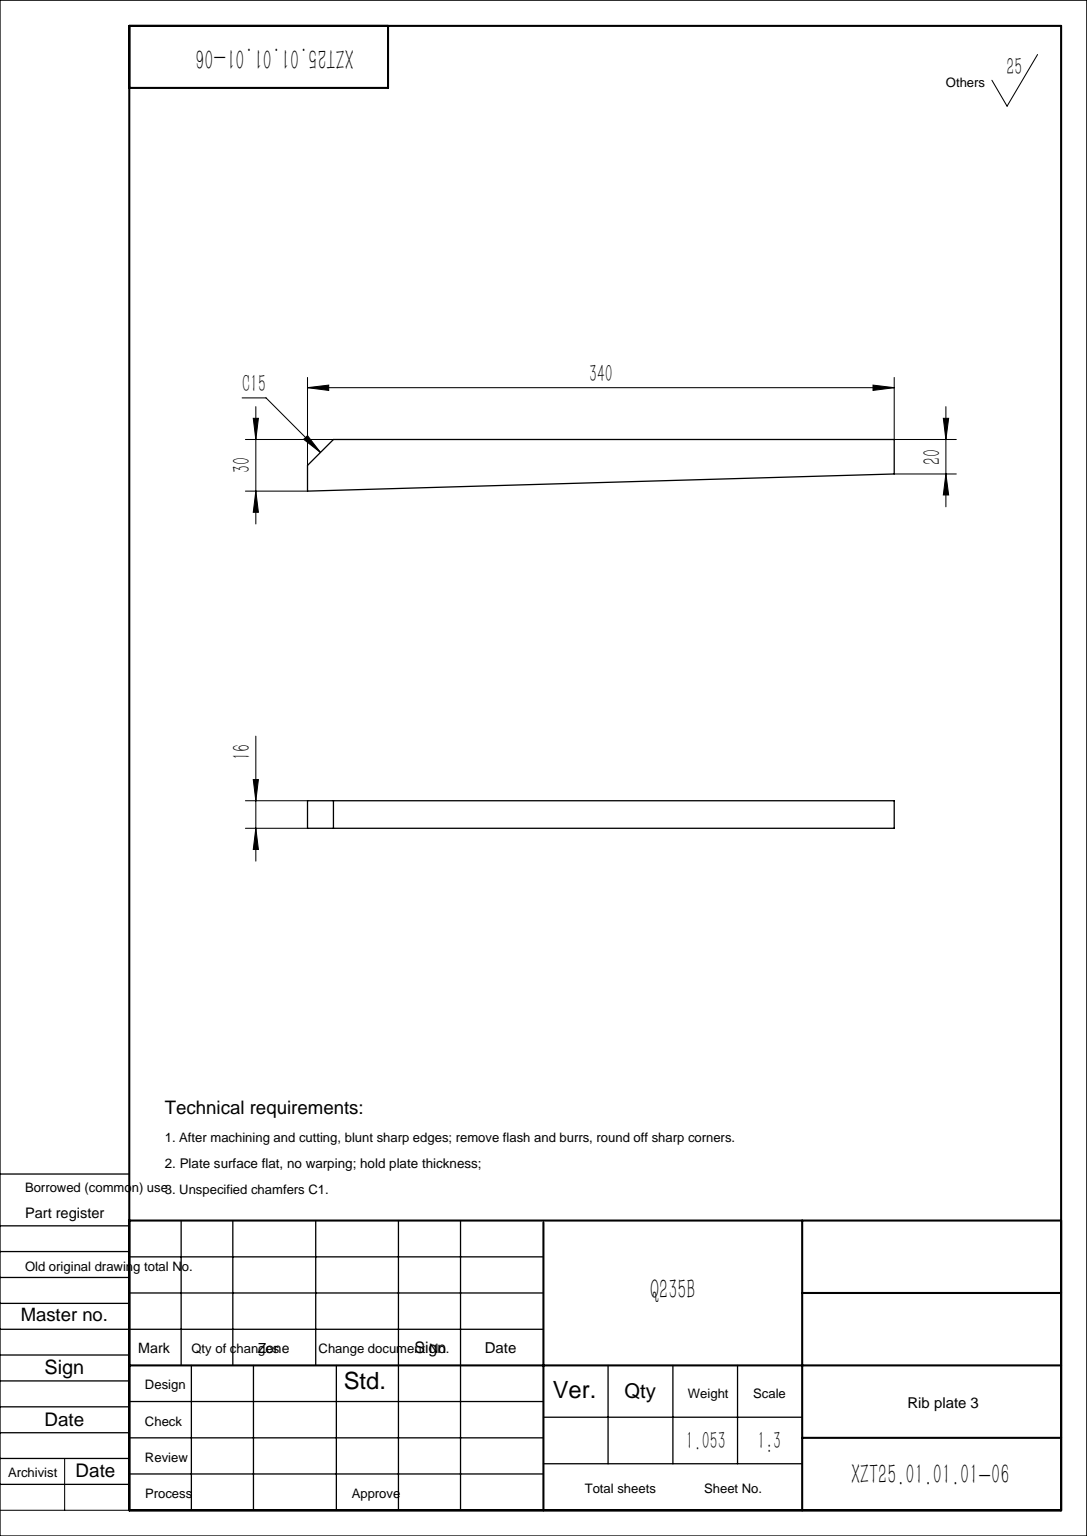
SolidWorks part; units mm, degrees
material "Q235B"
ref_plane "Front Plane" through (0, 0, 0) normal (0, 0, 1) x (1, 0, 0)
ref_plane "Top Plane" through (0, 0, 0) normal (0, 1, 0) x (1, 0, 0)
ref_plane "Right Plane" through (0, 0, 0) normal (1, 0, 0) x (0, 0, -1)
sketch "Sketch1" plane through (0, 0, 0) normal (0, 0, 1) x (1, 0, 0)
  line L0 (0, 0) -> (0, 30)
  line L1 (0, 30) -> (340, 30)
  line L2 (340, 30) -> (340, 10)
  line L3 (340, 10) -> (0, 0)
  dimension "D1" = 30
  dimension "D2" = 20
  dimension "D3" = 340
extrude "Boss-Extrude1" add sketch "Sketch1" along normal mid plane 16
chamfer "Chamfer1" distance 15 angle 45 1 edges at (0, 30, 0)
